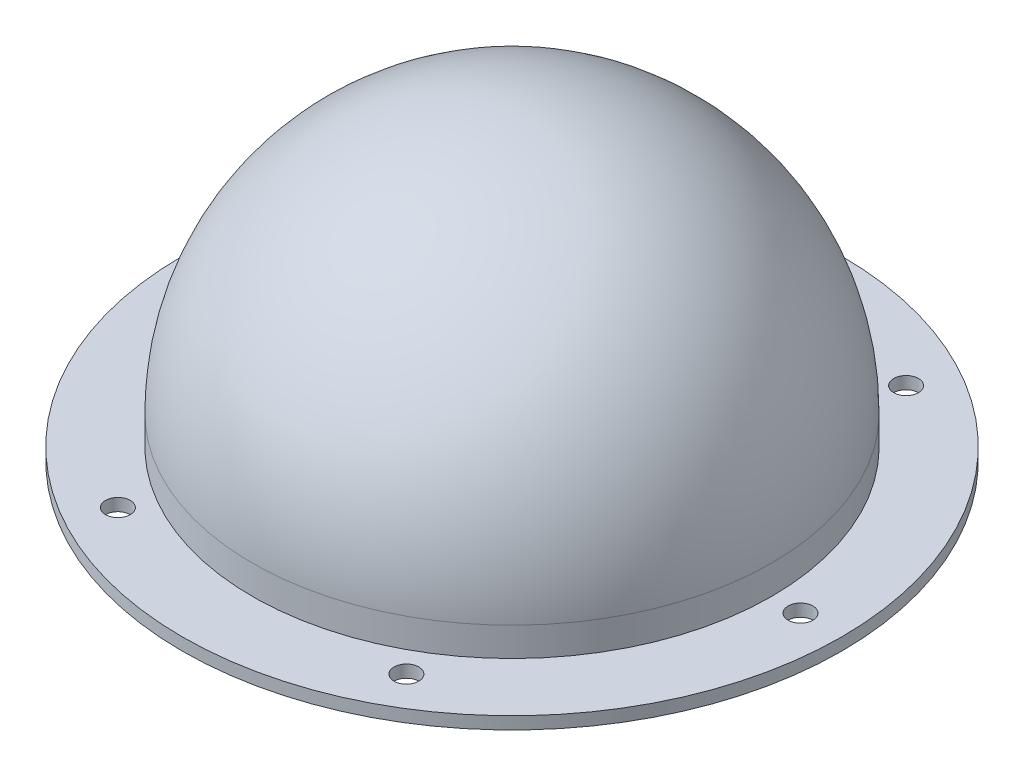
from build123d import *

# Parameters (mm, degrees)
SKETCH2_R          = 1.5
CUT_EXTRUDE1_DEPTH = 67.520673478


with BuildPart() as part:
    # Sketch1 → Revolve1 (revolve)
    with BuildSketch(Plane.XY, mode=Mode.PRIVATE) as revolve1_sk:
        with BuildLine():
            Line((-40, 0), (-30, 0))
            Line((-30, 0), (-30, 5))
            ThreePointArc((-30, 5), (-21.213203436, 26.213203436), (0, 35))
            Line((0, 35), (0, 36.5))
            ThreePointArc((0, 36.5), (-22.273863607, 27.273863607), (-31.5, 5))
            Line((-31.5, 5), (-31.5, 1.5))
            Line((-31.5, 1.5), (-40, 1.5))
            Line((-40, 1.5), (-40, 0))
        make_face()
    revolve(revolve1_sk.sketch.rotate(Axis((0, 35, 0), (0, 1, 0)), 180), axis=Axis((0, 35, 0), (0, 1, 0)))

    # Sketch2 → Cut-Extrude1 (cut, through all)
    with BuildSketch(Plane(origin=(0, 1.5, 0), x_dir=(1, 0, 0), z_dir=(0, 1, 0))):
        with Locations(Location((-35, 0, 0), (0, 0, 180))):
            Circle(SKETCH2_R)
        with Locations(Location((-17.5, 30.310889132, 0), (0, 0, 180))):
            Circle(SKETCH2_R)
        with Locations(Location((17.5, 30.310889132, 0), (0, 0, 180))):
            Circle(SKETCH2_R)
        with Locations(Location((35, 0, 0), (0, 0, 180))):
            Circle(SKETCH2_R)
        with Locations(Location((17.5, -30.310889132, 0), (0, 0, 180))):
            Circle(SKETCH2_R)
        with Locations(Location((-17.5, -30.310889132, 0), (0, 0, 180))):
            Circle(SKETCH2_R)
    extrude(amount=-CUT_EXTRUDE1_DEPTH, mode=Mode.SUBTRACT)


solid = part.part
